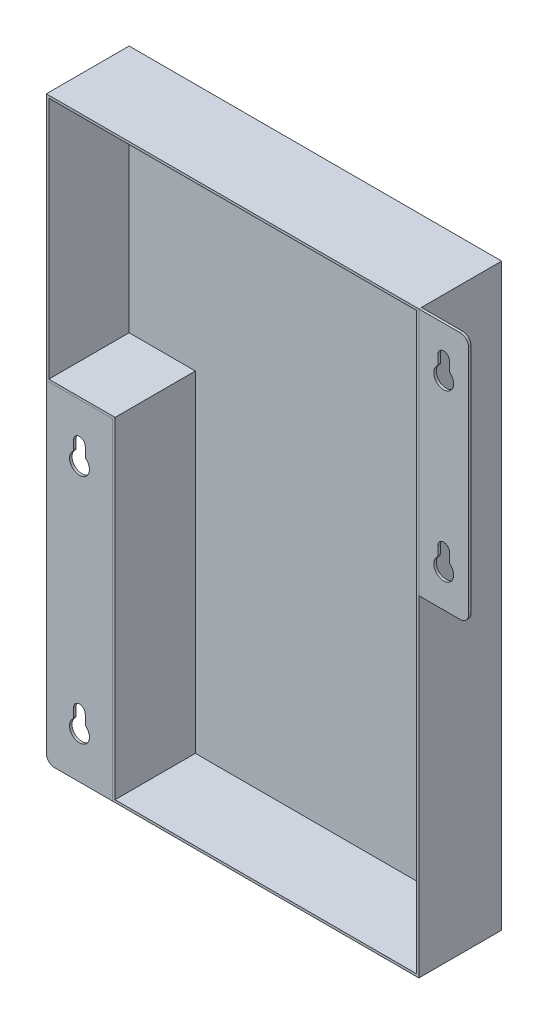
SolidWorks part; units mm, degrees
ref_plane "前视基准面" through (0, 0, 0) normal (0, 0, 1) x (1, 0, 0)
ref_plane "上视基准面" through (0, 0, 0) normal (0, 1, 0) x (1, 0, 0)
ref_plane "右视基准面" through (0, 0, 0) normal (1, 0, 0) x (0, 0, -1)
sketch "草图1" plane through (0, 0, 0) normal (0, 0, 1) x (1, 0, 0)
  line L1 (-112.5, 175) -> (112.5, 175)
  line L2 (-112.5, 175) -> (-112.5, -175)
  line L3 (-112.5, -175) -> (112.5, -175)
  line L4 (112.5, 175) -> (112.5, -175)
  line L5 (-112.5, 175) -> (112.5, -175) construction
  line L6 (-112.5, -175) -> (112.5, 175) construction
  point P0 (0, 0)
  dimension "D1" = 225
  dimension "D2" = 350
extrude "凸台-拉伸1" add sketch "草图1" along normal blind 50
sketch "草图2" plane through (0, 0, 0) normal (0, 0, -1) x (-1, 0, 0)
  line L1 (112.5, -175) -> (72.5, -175)
  line L2 (112.5, -175) -> (112.5, 25)
  line L3 (112.5, 25) -> (72.5, 25)
  line L4 (72.5, -175) -> (72.5, 25)
  dimension "D1" = 40
  dimension "D2" = 200
extrude "切除-拉伸1" cut sketch "草图2" against normal through all
shell "抽壳1" thickness 1.5
sketch "草图3" plane through (0, 0, 50) normal (0, 0, 1) x (1, 0, 0)
  line L1 (-72.5, -175) -> (-112.5, -175)
  line L2 (-72.5, -175) -> (-72.5, 25)
  line L3 (-72.5, 25) -> (-112.5, 25)
  line L4 (-112.5, -175) -> (-112.5, 25)
  line L6 (-112.5, 175) -> (-112.5, 25) construction
  line L8 (112.5, 175) -> (142.5, 175)
  line L9 (112.5, 175) -> (112.5, 25)
  line L10 (112.5, 25) -> (142.5, 25)
  line L11 (142.5, 175) -> (142.5, 25)
  dimension "D1" = 200
  dimension "D2" = 30
  dimension "D3" = 150
extrude "凸台-拉伸2" add sketch "草图3" against normal blind 1.5 separate body
fillet "圆角1" radius 5 2 edges at (142.5, 25, 49.25) (142.5, 175, 49.25)
fillet "圆角2" radius 5 1 edges at (-112.5, -175, 49.25)
sketch "草图4" plane through (0, 0, 0) normal (0, 0, -1) x (-1, 0, 0)
  line L0 (112.5, 25) -> (112.5, -170) construction
  line L1 (92.5, -8.5171) -> (92.5, -141) construction
  line L2 (107.5, -175) -> (72.5, -175) construction
  line L3 (-127.5, 146.1905) -> (-127.5, 46.1905) construction
  line L4 (-142.5, 30) -> (-142.5, 170) construction
  line L5 (-137.5, 175) -> (-112.5, 175) construction
  line B0 (92.5, 2.2924) -> (92.5, -1.7076) construction
  line B1 (96, 2.2924) -> (96, -2.7076)
  line B2 (89, 2.2924) -> (89, -2.7076)
  arc B3 (96, 2.2924) -> (89, 2.2924) centre (92.5, 2.2924) ccw
  arc B4 (88.375, -4.1599) -> (96.625, -4.1599) centre (92.5, -8.5171) ccw
  arc B5 (96, -2.7076) -> (96.625, -4.1599) centre (98, -2.7076) ccw
  arc B6 (89, -2.7076) -> (88.375, -4.1599) centre (87, -2.7076) cw
  line B7 (92.5, -137.7076) -> (72.5, -137.7076) construction
  line B8 (96, -137.7076) -> (96, -142.7076)
  line B9 (89, -137.7076) -> (89, -142.7076)
  arc B10 (96, -137.7076) -> (89, -137.7076) centre (92.5, -137.7076) ccw
  arc B11 (88.375, -144.1599) -> (96.625, -144.1599) centre (92.5, -148.5171) ccw
  arc B12 (96, -142.7076) -> (96.625, -144.1599) centre (98, -142.7076) ccw
  arc B13 (89, -142.7076) -> (88.375, -144.1599) centre (87, -142.7076) cw
  line B14 (-127.5, 157) -> (-147.5, 157) construction
  line B15 (-124, 157) -> (-124, 152)
  line B16 (-131, 157) -> (-131, 152)
  arc B17 (-124, 157) -> (-131, 157) centre (-127.5, 157) ccw
  arc B18 (-131.625, 150.5476) -> (-123.375, 150.5476) centre (-127.5, 146.1905) ccw
  arc B19 (-124, 152) -> (-123.375, 150.5476) centre (-122, 152) ccw
  arc B20 (-131, 152) -> (-131.625, 150.5476) centre (-133, 152) cw
  line B21 (-127.5, 57) -> (-147.5, 57) construction
  line B22 (-124, 57) -> (-124, 52)
  line B23 (-131, 57) -> (-131, 52)
  arc B24 (-124, 57) -> (-131, 57) centre (-127.5, 57) ccw
  arc B25 (-131.625, 50.5476) -> (-123.375, 50.5476) centre (-127.5, 46.1905) ccw
  arc B26 (-124, 52) -> (-123.375, 50.5476) centre (-122, 52) ccw
  arc B27 (-131, 52) -> (-131.625, 50.5476) centre (-133, 52) cw
  dimension "D1" = 20
  dimension "D2" = 32
  dimension "D3" = 140
  dimension "D4" = 15
  dimension "D5" = 18
  dimension "D6" = 100
sketch_block_instance "快拆孔-1"
sketch_block "快拆孔" parameters "D3"=12, "D4"=2, "D1"=20, "D2"=7, "D5"=3.0639
sketch_block_instance "快拆孔-3"
sketch_block_instance "快拆孔-5"
sketch_block_instance "快拆孔-6"
extrude "切除-拉伸4" cut sketch "草图4" against normal through all
